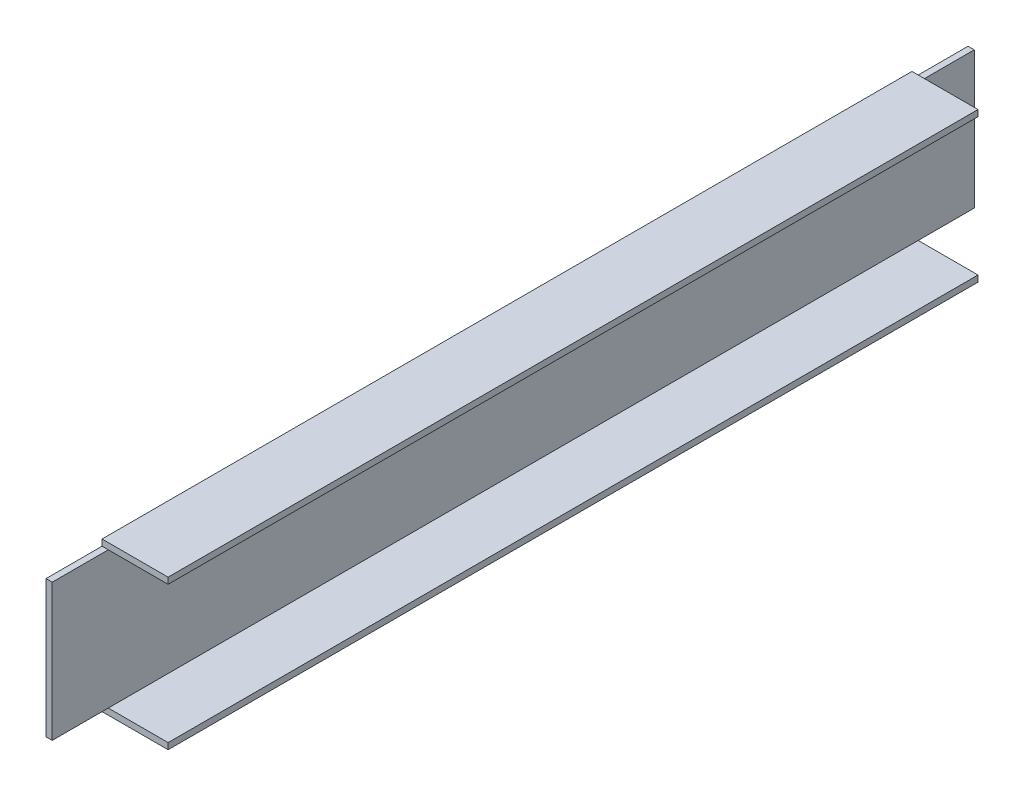
from build123d import *

# Parameters (mm, degrees)
EXTRUDE_1_DEPTH     = 740
SKETCH_2_W          = 53
SKETCH_2_H          = 5
CUT_EXTRUDE_1_DEPTH = 45
SKETCH_3_W          = 53
SKETCH_3_H          = 5
CUT_EXTRUDE_2_DEPTH = 45
SKETCH_4_W          = 53
SKETCH_4_H          = 5
CUT_EXTRUDE_3_DEPTH = 45


with BuildPart() as part:
    # 草图1 → 凸台-拉伸1 (new body)
    with BuildSketch(Plane.XY):
        Polygon((0, 0), (0, -120), (53, -120), (53, -115), (5, -115), (5, -5), (53, -5), (53, 0), align=None)
    extrude(amount=EXTRUDE_1_DEPTH)

    # 草图2 → 切除-拉伸1 (cut)
    with BuildSketch(Plane(origin=(0, 0, 0), x_dir=(-1, 0, 0), z_dir=(0, 0, -1))):
        with Locations((-26.5, -2.5)):
            Rectangle(SKETCH_2_W, SKETCH_2_H)
    extrude(amount=-CUT_EXTRUDE_1_DEPTH, mode=Mode.SUBTRACT)

    # 草图3 → 切除-拉伸2 (cut)
    with BuildSketch(Plane(origin=(0, 0, 0), x_dir=(-1, 0, 0), z_dir=(0, 0, -1))):
        with Locations((-26.5, -117.5)):
            Rectangle(SKETCH_3_W, SKETCH_3_H)
    extrude(amount=-CUT_EXTRUDE_2_DEPTH, mode=Mode.SUBTRACT)

    # 草图4 → 切除-拉伸3 (cut)
    with BuildSketch(Plane.XY.offset(740)):
        with Locations((26.5, -2.5)):
            Rectangle(SKETCH_4_W, SKETCH_4_H)
        with Locations((26.5, -117.5)):
            Rectangle(SKETCH_4_W, SKETCH_4_H)
    extrude(amount=-CUT_EXTRUDE_3_DEPTH, mode=Mode.SUBTRACT)


solid = part.part
